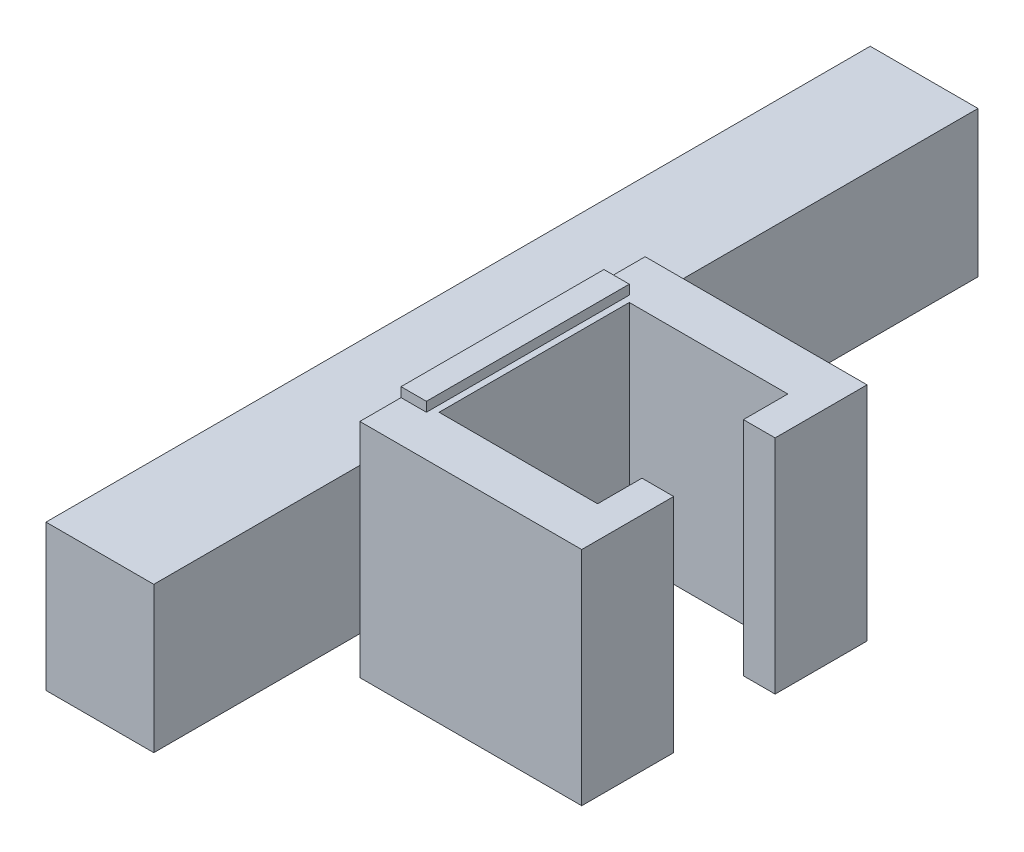
SolidWorks part; units mm, degrees
ref_plane "Front Plane" through (0, 0, 0) normal (0, 0, 1) x (1, 0, 0)
ref_plane "Top Plane" through (0, 0, 0) normal (0, 1, 0) x (1, 0, 0)
ref_plane "Right Plane" through (0, 0, 0) normal (1, 0, 0) x (0, 0, -1)
other "Configuration Table"
sketch "Sketch1" plane through (0, 0, 0) normal (0, 1, 0) x (1, 0, 0)
  line L0 (125, 80) -> (175, 80)
  line L1 (-125, 150) -> (125, 150)
  line L2 (-125, 150) -> (-125, -150)
  line L3 (-125, -150) -> (125, -150)
  line L4 (125, 150) -> (125, 80)
  line L5 (-125, 150) -> (125, -150) construction
  line L6 (-125, -150) -> (125, 150) construction
  line L7 (-175, 225) -> (175, 225)
  line L8 (-175, 225) -> (-175, -225)
  line L9 (-175, -225) -> (175, -225)
  line L10 (175, 225) -> (175, 80)
  line L11 (-175, 225) -> (175, -225) construction
  line L12 (-175, -225) -> (175, 225) construction
  line L13 (125, -80) -> (175, -80)
  line L14 (125, -80) -> (125, -150)
  line L15 (175, -80) -> (175, -225)
  point P0 (0, 0)
  point P6 (0, 0)
  dimension "D1" = 300
  dimension "D2" = 250
  dimension "D3" = 350
  dimension "D4" = 450
  dimension "D5" = 70
  dimension "D6" = 70
extrude "Boss-Extrude1" add sketch "Sketch1" along normal blind 350
sketch "Sketch2" plane through (-175, 0, 0) normal (-1, 0, 0) x (0, 0, 1)
  line L0 (0, 0) -> (0, 350) construction
  line L1 (-225, 0) -> (225, 0) construction
  line L2 (-225, 350) -> (225, 350) construction
  line L4 (-160, 365) -> (160, 365)
  line L5 (-160, 365) -> (-160, -15)
  line L6 (-160, -15) -> (160, -15)
  line L7 (160, 365) -> (160, -15)
  line L8 (-160, 365) -> (160, -15) construction
  line L9 (-160, -15) -> (160, 365) construction
  point P6 (0, 175)
  dimension "D1" = 320
  dimension "D2" = 380
extrude "Boss-Extrude2" add sketch "Sketch2" against normal blind 40
sketch "Sketch3" plane through (-175, 0, 0) normal (-1, 0, 0) x (0, 0, 1)
  line L0 (-225, 350) -> (225, 0) construction
  line L1 (225, 350) -> (225, 0) construction
  line L3 (-750, 290) -> (750, 290)
  line L4 (-750, 290) -> (-750, 60)
  line L5 (-750, 60) -> (750, 60)
  line L6 (750, 290) -> (750, 60)
  line L7 (-750, 290) -> (750, 60) construction
  line L8 (-750, 60) -> (750, 290) construction
  point P5 (0, 175)
  dimension "D1" = 1500
  dimension "D2" = 230
extrude "Boss-Extrude3" add sketch "Sketch3" along normal blind 170
sketch "Sketch5" plane through (0, 0, 750) normal (0, 0, 1) x (1, 0, 0)
  line L1 (-360.42, 331.8811) -> (-140.3181, 331.8811)
  line L2 (-360.42, 331.8811) -> (-360.42, 22.8019)
  line L3 (-360.42, 22.8019) -> (-140.3181, 22.8019)
  line L4 (-140.3181, 331.8811) -> (-140.3181, 22.8019)
  line L5 (-360.42, 331.8811) -> (-140.3181, 22.8019) construction
  line L6 (-360.42, 22.8019) -> (-140.3181, 331.8811) construction
  point P0 (-250.369, 177.3415)
extrude "Cut-Extrude2" cut sketch "Sketch5" against normal blind 200
ref_plane "Plane1" through (0, 0, -735) normal (0, 0, -1) x (-1, 0, 0)
sketch "Sketch6" plane through (0, 0, -735) normal (0, 0, -1) x (-1, 0, 0)
  line L0 (175, 175) -> (545.8709, 175) construction
  line L1 (175, 290) -> (175, 60) construction
  line L2 (345, 290) -> (345, 60) construction
  line L3 (346, 215) -> (376, 215)
  line L4 (346, 215) -> (346, 135)
  line L5 (346, 135) -> (376, 135)
  line L6 (396, 215) -> (396, 135)
  line L7 (346, 215) -> (396, 135) construction
  line L8 (346, 135) -> (396, 215) construction
  line L9 (376, 215) -> (376, 200)
  line L10 (376, 200) -> (386, 200)
  line L11 (386, 200) -> (386, 215)
  line L12 (386, 135) -> (386, 150)
  line L13 (386, 150) -> (376, 150)
  line L14 (376, 150) -> (376, 135)
  line L15 (386, 215) -> (396, 215)
  line L16 (386, 135) -> (396, 135)
  point P4 (371, 175)
  dimension "D1" = 1
  dimension "D2" = 50
  dimension "D3" = 80
  dimension "D4" = 10
  dimension "D5" = 10
  dimension "D6" = 15
  dimension "D7" = 15
  dimension "D8" = 10
extrude "Boss-Extrude4" add sketch "Sketch6" against normal blind 1170 separate body
